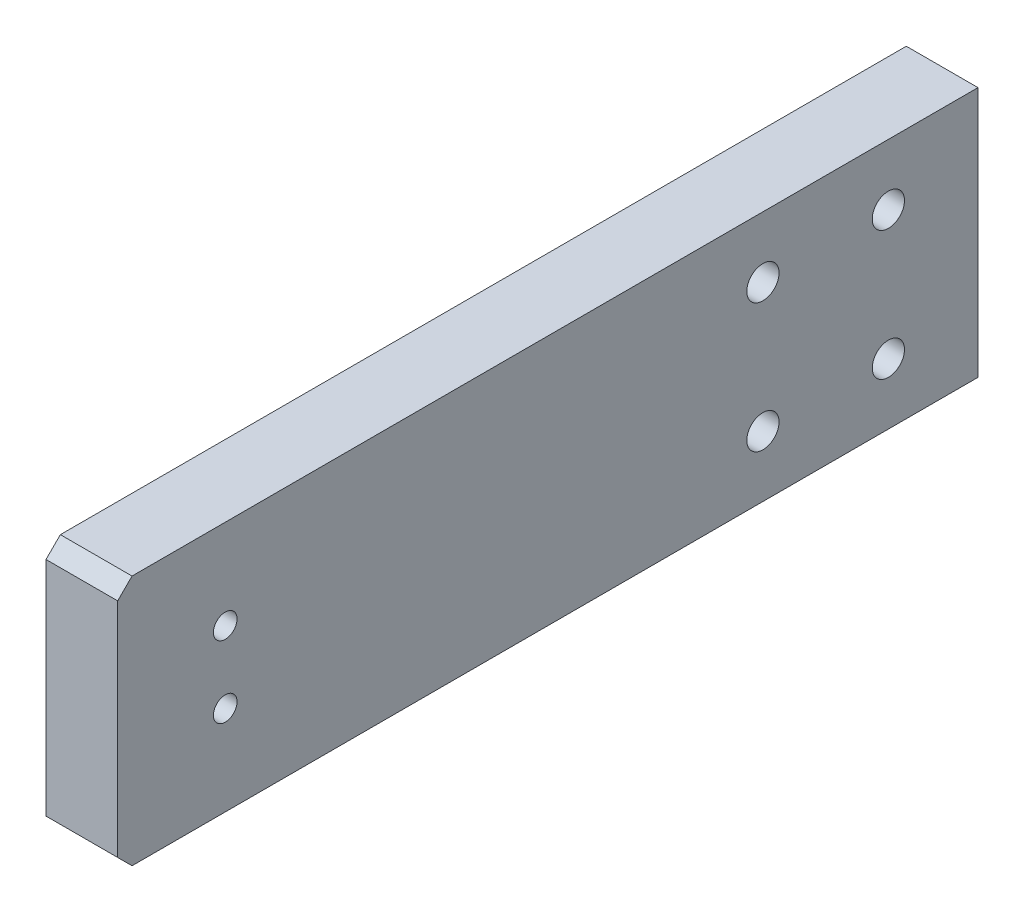
SolidWorks part; units mm, degrees
material "电木（PF）"
ref_plane "前视基准面" through (0, 0, 0) normal (0, 0, 1) x (1, 0, 0)
ref_plane "上视基准面" through (0, 0, 0) normal (0, 1, 0) x (1, 0, 0)
ref_plane "右视基准面" through (0, 0, 0) normal (1, 0, 0) x (0, 0, -1)
sketch "草图1" plane through (0, 0, 0) normal (1, 0, 0) x (0, 0, -1)
  line L1 (-60, 17.5) -> (60, 17.5)
  line L2 (-60, 17.5) -> (-60, -17.5)
  line L3 (-60, -17.5) -> (60, -17.5)
  line L4 (60, 17.5) -> (60, -17.5)
  line L5 (-60, 17.5) -> (60, -17.5) construction
  line L6 (-60, -17.5) -> (60, 17.5) construction
  point P0 (0, 0)
  dimension "D1" = 120
  dimension "D2" = 35
extrude "凸台-拉伸1" add sketch "草图1" along normal blind 10
hole_wizard "M4 螺纹孔1" positions "草图2" profile "草图4" tap size "M4" standard "GB" end condition through all
sketch "草图2" plane through (0, 0, 0) normal (-1, 0, 0) x (0, 0, 1)
  line L0 (0, 0) -> (-53.6018, 0) construction
  line L3 (60, 17.5) -> (60, -17.5) construction
  point P0 (45, 5)
  point P7 (45, -5)
  dimension "D1" = 10
  dimension "D2" = 15
sketch "草图4" plane through (0, 5, 45) normal (0, 1, 0) x (0, 0, 1)
  line L0 (0, 0) -> (0, 10)
  line L1 (0, 10) -> (1.65, 10)
  line L2 (1.65, 10) -> (1.65, 0)
  line L5 (1.65, 0) -> (0, 0)
  line L11 (0, -6.35) -> (0, 107.95) construction
  dimension "通孔螺纹孔钻头直径" = 3.3
  dimension "通孔螺纹孔钻头深度" = 10
cosmetic thread "孔螺蚊线1" parameters "D2"=4
cosmetic thread "孔螺蚊线2" parameters "D2"=4
sketch "草图5" plane through (0, 0, 0) normal (-1, 0, 0) x (0, 0, 1)
  line L0 (0, 0) -> (-51.6304, 0) construction
  line L1 (-60, -17.5) -> (-60, 17.5) construction
  circle A0 centre (-47.5, 9) radius 2.25
  circle A1 centre (-47.5, -9) radius 2.25
  dimension "D2" = 12.5
  dimension "D3" = 4.5
  dimension "D1" = 18
extrude "切除-拉伸1" cut sketch "草图5" against normal blind 28
chamfer "倒角1" distance 2 angle 45 2 edges at (5, -17.5, 60) (5, 17.5, 60)
pattern_linear "阵列(线性)1" count 2 spacing 17.5 along (0, 0, 1) of "切除-拉伸1"
